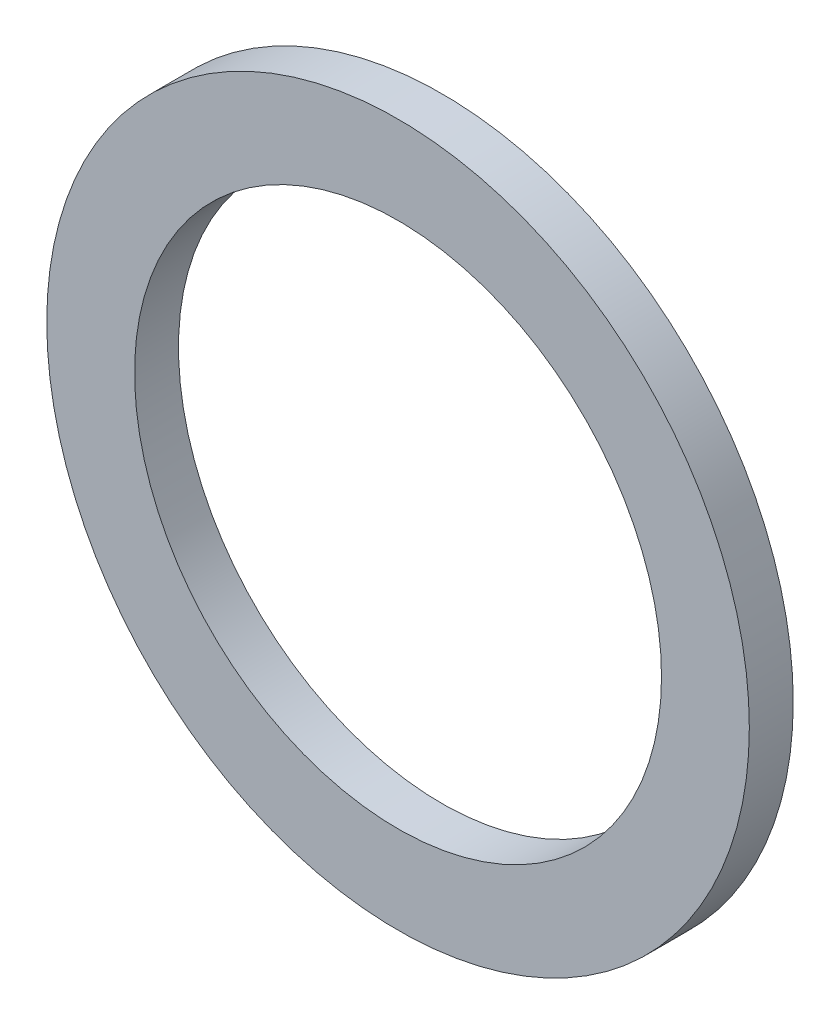
from build123d import *

# Parameters (mm, degrees)
SKETCH1_R           = 8
SKETCH1_R_2         = 6
BOSS_EXTRUDE1_DEPTH = 1


with BuildPart() as part:
    # Sketch1 → Boss-Extrude1 (new body)
    with BuildSketch(Plane.XY):
        Circle(SKETCH1_R)
        Circle(SKETCH1_R_2, mode=Mode.SUBTRACT)
    extrude(amount=BOSS_EXTRUDE1_DEPTH)


solid = part.part
